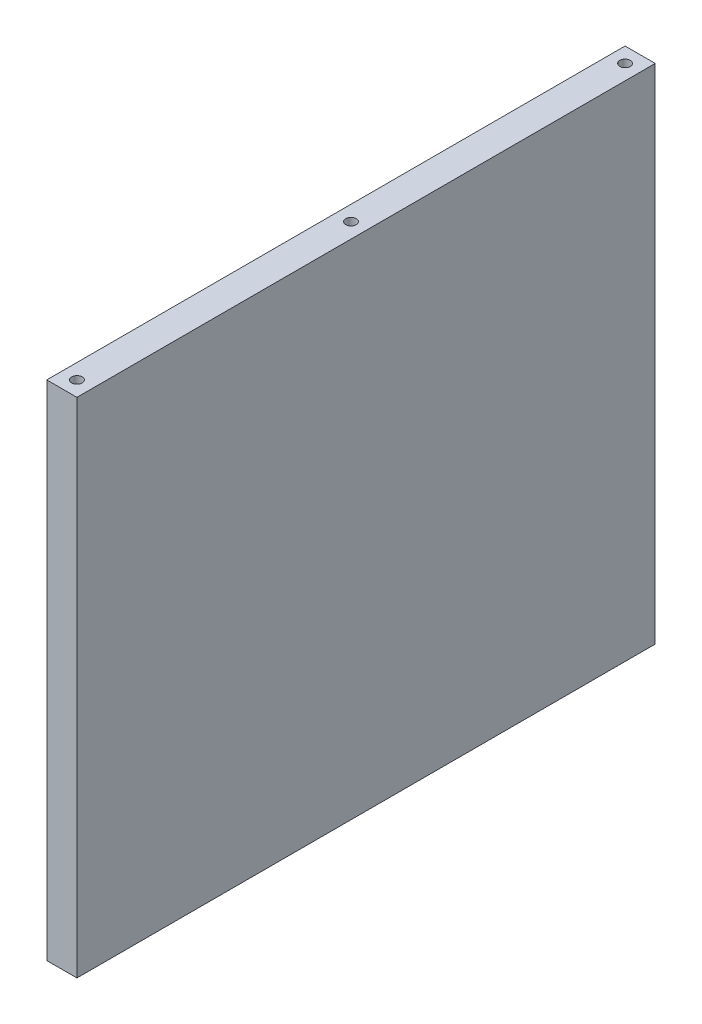
SolidWorks part; units mm, degrees
material "国产6061 "
ref_plane "Front Plane" through (0, 0, 0) normal (0, 0, 1) x (1, 0, 0)
ref_plane "Top Plane" through (0, 0, 0) normal (0, 1, 0) x (1, 0, 0)
ref_plane "Right Plane" through (0, 0, 0) normal (1, 0, 0) x (0, 0, -1)
sketch "Sketch1" plane through (0, 0, 0) normal (1, 0, 0) x (0, 0, -1)
  line L1 (-115, 100) -> (115, 100)
  line L2 (-115, 100) -> (-115, -100)
  line L3 (-115, -100) -> (115, -100)
  line L4 (115, 100) -> (115, -100)
  line L5 (-115, 100) -> (115, -100) construction
  line L6 (-115, -100) -> (115, 100) construction
  point P0 (0, 0)
  dimension "D1" = 200
  dimension "D2" = 230
extrude "Boss-Extrude1" add sketch "Sketch1" along normal mid plane 12
hole_wizard "M5 Tapped Hole1" positions "Sketch2" profile "Sketch3" tap size "M5" standard "GB"
sketch "Sketch2" plane through (0, 100, 0) normal (0, 1, 0) x (1, 0, 0)
  line L0 (6, 115) -> (-6, 115) construction
  line L1 (6, -115) -> (-6, -115) construction
  point P0 (0, 109)
  point P2 (0, 0)
  point P5 (0, -109)
  dimension "D1" = 6
  dimension "D2" = 6
sketch "Sketch3" plane through (0, 100, -109) normal (1, 0, 0) x (0, 0, 1)
  line L0 (0, 0) -> (0, 25.7618)
  line L1 (0, 25.7618) -> (2.1, 24.5)
  line L2 (2.1, 24.5) -> (2.1, 0)
  line L5 (2.1, 0) -> (0, 0)
  line L10 (0, 25.7618) -> (-2.1, 24.5) construction
  line L11 (0, -6.35) -> (0, 107.95) construction
  dimension "螺纹孔钻头直径" = 4.2
  dimension "螺纹孔钻头深度" = 24.5
  dimension "导头角度" = 118
cosmetic thread "Cosmetic thread 1" parameters "D1"=10, "D2"=5
cosmetic thread "Cosmetic thread 2" parameters "D1"=10, "D2"=5
cosmetic thread "Cosmetic thread 3" parameters "D1"=10, "D2"=5
mirror "Mirror1" about plane through (0, 0, 0) normal (0, 1, 0) of "M5 Tapped Hole1"
